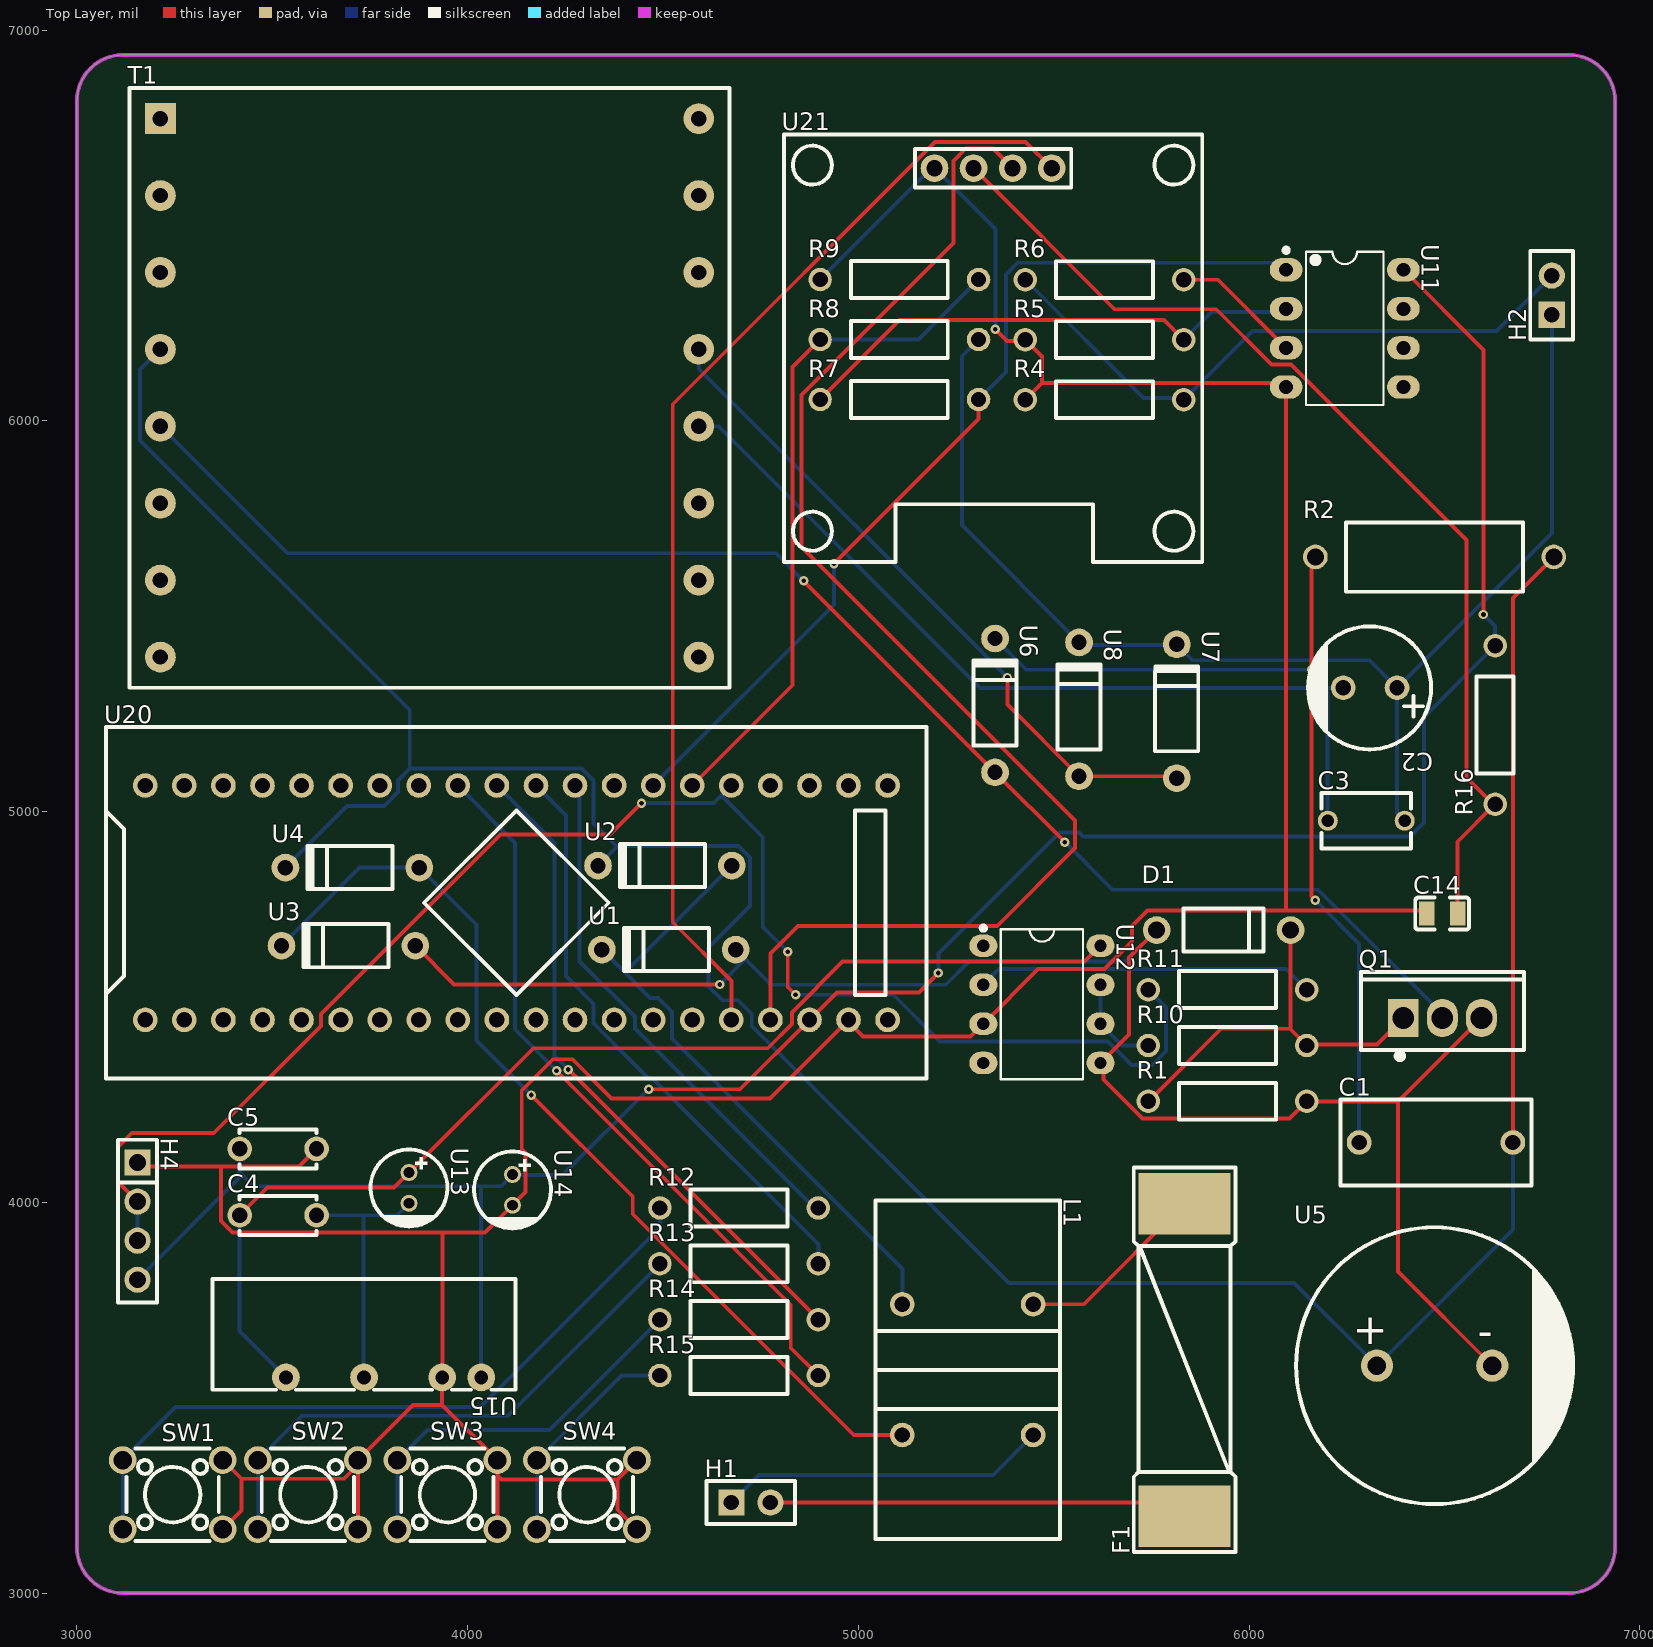
[diagram p0: Top Layer view]
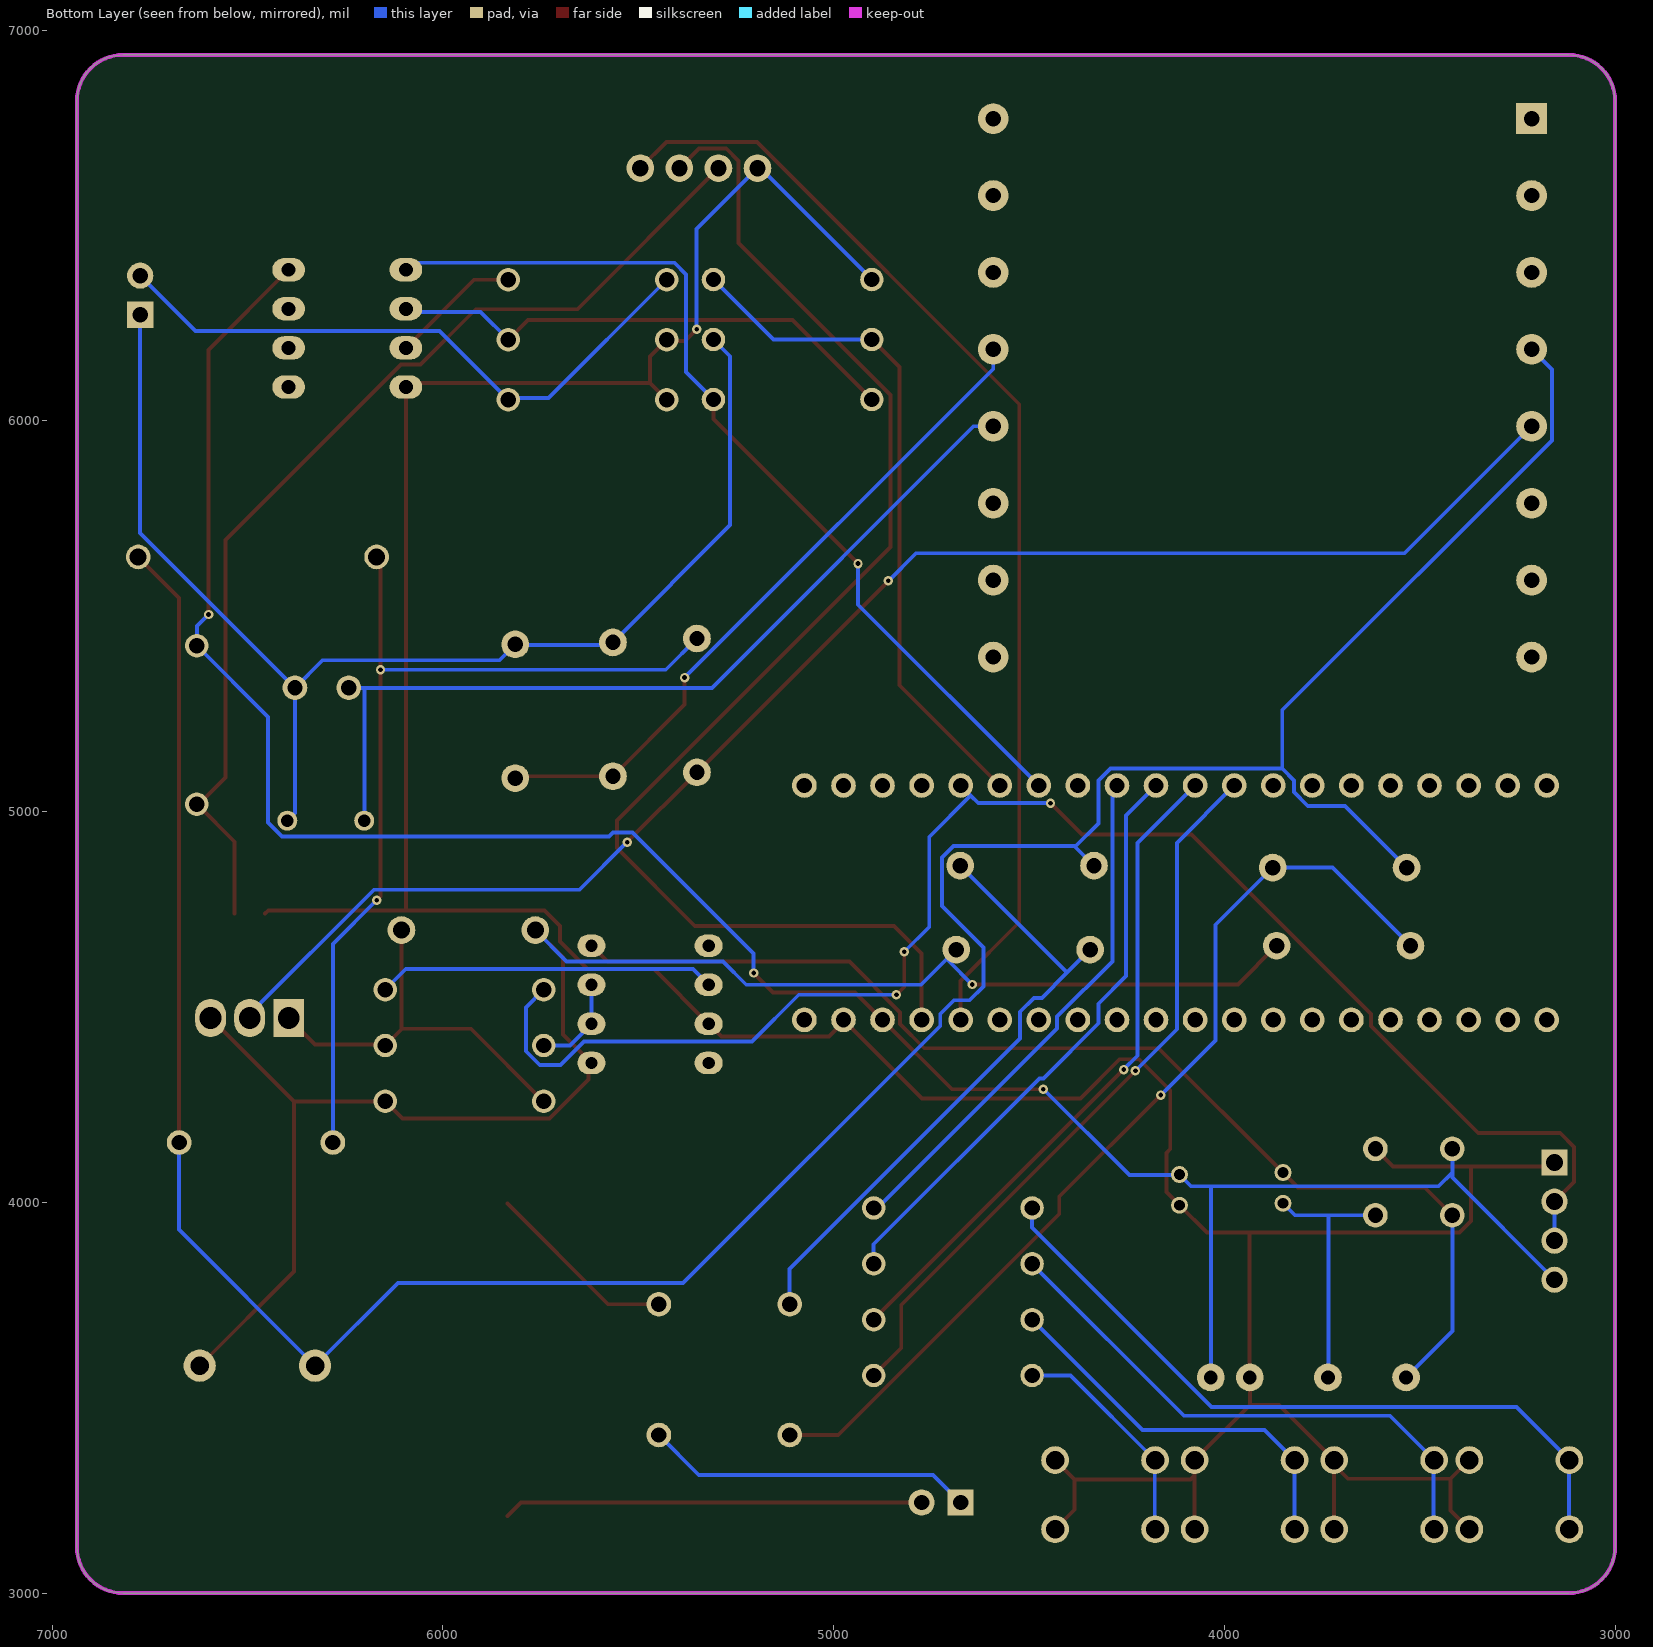
[diagram p1: Bottom Layer view, seen from below]
# Altium PCB MISC75075.pcbdoc
Units mil, origin at the board's own origin, x right, y up, seen from the top; angles counter-clockwise.
Board outline 3937.01 x 3937.01 mil, 2 copper layers (Top Layer, Bottom Layer), stack 62.206 mil thick; 48 components, 60 nets, 177 pads, 17 vias.

## Layer stack, top to bottom
Top Solder Mask Layer: solder mask 0.394, Dk 3.3
Top Layer: signal copper 1.379
Dielectric1: surface 59.449, FR4, Dk 4.5
Bottom Layer: signal copper 1.378
Bottom Solder Mask Layer: solder mask 0.394, Dk 3.3

## Board outline
3118.11,6937.01 ccw(c3118.11,6818.9) 3000,6818.9 3000,3118.11 ccw(c3118.11,3118.11) 3118.11,3000 6818.9,3000 ccw(c6818.9,3118.11) 6937.01,3118.11 6937.01,6818.9 ccw(c6818.9,6818.9) 6818.9,6937.01 3118.11,6937.01

## Design rules (kind name [scope] priority, off if disabled: settings)
BoardOutlineClearance copperThickness2oz_1 [All] p2 off: genericclearance=7.99 ignorepadtopadclearanceinfootprint=FALSE except(0: Arc-SplitContinuation Track-SplitContinuation SMDPad-SplitContinuation THPad-SplitContinuation Via-SplitContinuation Fill-SplitContinuation Region-SplitContinuation Poly-SplitContinuation Text-SplitContinuation Hole-SplitContinuation; 5.98: Arc-CutoutEdge Track-CutoutEdge SMDPad-CutoutEdge THPad-CutoutEdge Via-CutoutEdge Text-CutoutEdge; 6.9: Hole-OutlineEdge Hole-CutoutEdge; 10: Poly-OutlineEdge Poly-CutoutEdge; 11.81: Arc-OutlineEdge Track-OutlineEdge SMDPad-OutlineEdge THPad-OutlineEdge Via-OutlineEdge Fill-OutlineEdge Region-OutlineEdge Text-OutlineEdge Fill-CutoutEdge Region-CutoutEdge)
BoardOutlineClearance Plane_innerPlane_1 [All] p4 off: genericclearance=4.02 ignorepadtopadclearanceinfootprint=FALSE except(0: Arc-SplitContinuation Track-SplitContinuation SMDPad-SplitContinuation THPad-SplitContinuation Via-SplitContinuation Fill-SplitContinuation Region-SplitContinuation Poly-SplitContinuation Text-SplitContinuation Hole-SplitContinuation; 5.98: Arc-CutoutEdge Track-CutoutEdge SMDPad-CutoutEdge THPad-CutoutEdge Via-CutoutEdge Text-CutoutEdge; 6.9: Hole-OutlineEdge Hole-CutoutEdge; 10: Poly-OutlineEdge Poly-CutoutEdge; 11.81: Arc-OutlineEdge Track-OutlineEdge SMDPad-OutlineEdge THPad-OutlineEdge Via-OutlineEdge Fill-OutlineEdge Region-OutlineEdge Text-OutlineEdge Fill-CutoutEdge Region-CutoutEdge)
BoardOutlineClearance Copper_copperRegion_1 [All] p6 off: genericclearance=4.02 ignorepadtopadclearanceinfootprint=FALSE except(0: Arc-SplitContinuation Track-SplitContinuation SMDPad-SplitContinuation THPad-SplitContinuation Via-SplitContinuation Fill-SplitContinuation Region-SplitContinuation Poly-SplitContinuation Text-SplitContinuation Hole-SplitContinuation; 5.98: Arc-CutoutEdge Track-CutoutEdge SMDPad-CutoutEdge THPad-CutoutEdge Via-CutoutEdge Text-CutoutEdge; 6.9: Hole-OutlineEdge Hole-CutoutEdge; 10: Poly-OutlineEdge Poly-CutoutEdge; 11.81: Arc-OutlineEdge Track-OutlineEdge SMDPad-OutlineEdge THPad-OutlineEdge Via-OutlineEdge Fill-OutlineEdge Region-OutlineEdge Text-OutlineEdge Fill-CutoutEdge Region-CutoutEdge)
BoardOutlineClearance copperThickness1oz_1 [All] p8: genericclearance=4.02 ignorepadtopadclearanceinfootprint=FALSE except(0: Arc-SplitContinuation Track-SplitContinuation SMDPad-SplitContinuation THPad-SplitContinuation Via-SplitContinuation Fill-SplitContinuation Region-SplitContinuation Poly-SplitContinuation Text-SplitContinuation Hole-SplitContinuation; 5.98: Arc-CutoutEdge Track-CutoutEdge SMDPad-CutoutEdge THPad-CutoutEdge Via-CutoutEdge Text-CutoutEdge; 6.9: Hole-OutlineEdge Hole-CutoutEdge; 10: Poly-OutlineEdge Poly-CutoutEdge; 11.81: Arc-OutlineEdge Track-OutlineEdge SMDPad-OutlineEdge THPad-OutlineEdge Via-OutlineEdge Fill-OutlineEdge Region-OutlineEdge Text-OutlineEdge Fill-CutoutEdge Region-CutoutEdge)
Clearance copperThickness2oz [All] p1 off: gap=7.99 ignorepadtopadclearanceinfootprint=FALSE except(5.98: SMDPad-Track SMDPad-SMDPad THPad-Track SMDPad-THPad THPad-THPad Track-Via SMDPad-Via THPad-Via Via-Via Fill-SMDPad Region-SMDPad Fill-THPad Region-THPad Fill-Via Region-Via Fill-Fill Fill-Region Region-Region Arc-Track Arc-SMDPad Arc-THPad Arc-Via Fill-Arc Region-Arc Arc-Arc Text-Track SMDPad-Text Text-THPad Text-Via Fill-Text Region-Text Arc-Text Text-Text; 6.9: Hole-Track Hole-SMDPad Hole-THPad Hole-Via Fill-Hole Region-Hole Hole-Arc Hole-Text; 10: Poly-Track Poly-SMDPad Poly-THPad Poly-Via Poly-Fill Poly-Region Poly-Poly Poly-Arc Poly-Text Poly-Hole; 11.81: Fill-Track Region-Track)
Clearance Plane_innerPlane [All] p3 off: gap=4.02 ignorepadtopadclearanceinfootprint=FALSE except(5.98: SMDPad-Track SMDPad-SMDPad THPad-Track SMDPad-THPad THPad-THPad Track-Via SMDPad-Via THPad-Via Via-Via Fill-SMDPad Region-SMDPad Fill-THPad Region-THPad Fill-Via Region-Via Fill-Fill Fill-Region Region-Region Arc-Track Arc-SMDPad Arc-THPad Arc-Via Fill-Arc Region-Arc Arc-Arc Text-Track SMDPad-Text Text-THPad Text-Via Fill-Text Region-Text Arc-Text Text-Text; 6.9: Hole-Track Hole-SMDPad Hole-THPad Hole-Via Fill-Hole Region-Hole Hole-Arc Hole-Text; 10: Poly-Track Poly-SMDPad Poly-THPad Poly-Via Poly-Fill Poly-Region Poly-Poly Poly-Arc Poly-Text Poly-Hole; 11.81: Fill-Track Region-Track)
Clearance Copper_copperRegion [All] p5 off: gap=4.02 ignorepadtopadclearanceinfootprint=FALSE except(5.98: SMDPad-Track SMDPad-SMDPad THPad-Track SMDPad-THPad THPad-THPad Track-Via SMDPad-Via THPad-Via Via-Via Fill-SMDPad Region-SMDPad Fill-THPad Region-THPad Fill-Via Region-Via Fill-Fill Fill-Region Region-Region Arc-Track Arc-SMDPad Arc-THPad Arc-Via Fill-Arc Region-Arc Arc-Arc Text-Track SMDPad-Text Text-THPad Text-Via Fill-Text Region-Text Arc-Text Text-Text; 6.9: Hole-Track Hole-SMDPad Hole-THPad Hole-Via Fill-Hole Region-Hole Hole-Arc Hole-Text; 10: Poly-Track Poly-SMDPad Poly-THPad Poly-Via Poly-Fill Poly-Region Poly-Poly Poly-Arc Poly-Text Poly-Hole; 11.81: Fill-Track Region-Track)
Clearance copperThickness1oz [All] p7: gap=4.02 ignorepadtopadclearanceinfootprint=FALSE except(5.98: SMDPad-Track SMDPad-SMDPad THPad-Track SMDPad-THPad THPad-THPad Track-Via SMDPad-Via THPad-Via Via-Via Fill-SMDPad Region-SMDPad Fill-THPad Region-THPad Fill-Via Region-Via Fill-Fill Fill-Region Region-Region Arc-Track Arc-SMDPad Arc-THPad Arc-Via Fill-Arc Region-Arc Arc-Arc Text-Track SMDPad-Text Text-THPad Text-Via Fill-Text Region-Text Arc-Text Text-Text; 6.9: Hole-Track Hole-SMDPad Hole-THPad Hole-Via Fill-Hole Region-Hole Hole-Arc Hole-Text; 10: Poly-Track Poly-SMDPad Poly-THPad Poly-Via Poly-Fill Poly-Region Poly-Poly Poly-Arc Poly-Text Poly-Hole; 11.81: Fill-Track Region-Track)
DiffPairsRouting differentialPair [All] p1: maxlimit=6 minlimit=6 mostfreqgap=6 toplayer_minwidth=5 toplayer_prefwidth=10 toplayer_maxwidth=100 toplayer_mingap=6 toplayer_prefgap=6 toplayer_maxgap=6 bottomlayer_minwidth=5 bottomlayer_prefwidth=10 bottomlayer_maxwidth=100 bottomlayer_mingap=6 bottomlayer_prefgap=6 bottomlayer_maxgap=6 maxuncoupledlength=10
HoleToHoleClearance otherClearance [All] p1: gap=11.81 allowstackedmicrovias=TRUE
Length netLength [All] p1: minlimit=0 maxlimit=0
PasteMaskExpansion pasteMaskExpansion [All] p1: expansion=0
PlaneConnect innerPlane [All] p1: planeconnectstyle=Relief reliefexpansion=20 reliefentries=4 reliefconductorwidth=10 reliefairgap=10
PolygonConnect copperRegion [All] p1: connectstyle=Relief reliefconductorwidth=10 reliefentries=4 polygonreliefangle="90 Angle" airgapwidth=10 via.connectstyle=Relief via.reliefconductorwidth=10 via.reliefentries=4 via.polygonreliefangle="90 Angle" via.airgapwidth=10
RoutingVias viaSize [All] p1: holewidth=12.01 width=24.02 viastyle="Through Hole" minholewidth=11.81 minwidth=19.68 maxholewidth=248.03 maxwidth=393.7
SolderMaskExpansion solderMaskExpansion [IsVia] p1: expansion=-1000 istentingtop=TRUE
SolderMaskExpansion solderMaskExpansion [All] p2: expansion=2 istentingtop=FALSE
Width copperThickness2oz_2 [All] p1 off: maxlimit=100 minlimit=8 preferedwidth=10
Width copperThickness1oz_2 [All] p2: maxlimit=100 minlimit=5 preferedwidth=10

## Components (designator, comment, footprint, x,y, rotation, side; value= is the part's Value field where it differs from the comment)
C1 "100uF" CAP-TH_L12.0-W5.5-P10.00-D1.0 6478.63,4153.38 r0 top
C2 "220uF" CAP-TH_BD8.0-P3.50-D0.6-FD 6310,5317.01 r180 top
C3 "1uF" CAP-TH_L5.8-W3.6-P5.0-D0.6 6300,4977.01 r0 top
C4 "100nF" CAP-TH_L5.0-W2.5-P5.00-D1.0 3515,3967.01 r0 top
C5 "100nF" CAP-TH_L5.0-W2.5-P5.00-D1.0 3515,4137.01 r0 top
C14 "100nF" C0805 6494.43,4739.12 r0 top
D1 "1N4742" DO-41_BD2.4-L4.7-P8.70-D0.8-FD 5935,4697.01 r0 top
F1 "5F.2000210000R1" FUSE-SMD_5-20MM 5835,3597.01 r90 top
H1 "" HDR-TH_2P-P2.54-V-F 4725,3232.01 r0 top
H2 "" HDR-TH_2P-P2.54-V-F 6775,6322.01 r90 top
H4 "" HDR-TH_4P-P2.54-V-F 3155,3952.01 r270 top
L1 "PDMCAT18107-103ML" IND-TH_4P-L22.0-W12.0-TR 5280,3572.01 r270 top
Q1 "FQPF8N60C" TO-220F-3_L10.2-W4.9-P2.54-L 6495,4472.01 r0 top
R1 "10kΩ" Res_1/4W 5945,4258.67 r0 top
R2 "10kΩ" Res_1W 6475,5652.01 r0 top
R4 "10mΩ" Res_1/4W 5630,6054.51 r0 top
R5 "2kΩ" Res_1/4W 5630,6208.01 r0 top
R6 "2kΩ" Res_1/4W 5630,6361.51 r0 top
R7 "200kΩ" Res_1/4W 5105,6055.01 r0 top
R8 "10kΩ" Res_1/4W 5105,6208.51 r0 top
R9 "2kΩ" Res_1/4W 5105,6362.01 r0 top
R10 "10Ω" Res_1/4W 5945,4401.59 r0 top
R11 "1kΩ" Res_1/4W 5945,4544.51 r0 top
R12 "2kΩ" Res_1/4W 4695,3985.76 r0 top
R13 "2kΩ" Res_1/4W 4695,3842.84 r0 top
R14 "2kΩ" Res_1/4W 4695,3699.92 r0 top
R15 "2kΩ" Res_1/4W 4695,3557.01 r0 top
R16 "1kΩ" Res_1/4W 6630,5222.01 r90 top
SW1 "TS-1002-07026" SW-TH_4P-L6.0-W6.0-P4.50-LS6.5 3245,3252.01 r0 top
SW2 "TS-1002-07026" SW-TH_4P-L6.0-W6.0-P4.50-LS6.5 3591.17,3252.01 r0 top
SW3 "TS-1002-07026" SW-TH_4P-L6.0-W6.0-P4.50-LS6.5 3948.33,3252.01 r0 top
SW4 "TS-1002-07026" SW-TH_4P-L6.0-W6.0-P4.50-LS6.5 4305.5,3252.01 r0 top
T1 "" dip2_8_5mm_35MM 3135,6577.01 r0 top
U1 "1N4007" DO-41_BD2.4-L4.7-P8.70-D0.6-RD 4515,4647.01 r0 top
U2 "1N4007" DO-41_BD2.4-L4.7-P8.70-D0.6-RD 4505,4862.01 r0 top
U3 "1N4007" DO-41_BD2.4-L4.7-P8.70-D0.6-RD 3695,4657.01 r0 top
U4 "1N4007" DO-41_BD2.4-L4.7-P8.70-D0.6-RD 3705,4857.01 r0 top
U5 "150uF" CAP-TH_BD18.0-P7.50-D0.8-FD 6475,3582.01 r0 top
U6 "1N4007" DO-41_BD2.4-L4.7-P8.70-D0.6-RD 5350,5272.01 r270 top
U7 "1N4007" DO-41_BD2.4-L4.7-P8.70-D0.6-RD 5815,5257.01 r270 top
U8 "1N4007" DO-41_BD2.4-L4.7-P8.70-D0.6-RD 5565,5262.01 r270 top
U11 "LM358" DIP-8_L9.8-W6.4-P2.54-LS7.6-BL 6245,6237.01 r270 top
U12 "TLP250(F)" DIP-8_L9.4-W6.4-P2.54-LS9.1-BL 5470,4507.01 r270 top
U13 "47uF" CAP-TH_BD5.0-P2.00-D0.5-FD 3850,4037.01 r270 top
U14 "100uF" CAP-TH_BD5.0-P2.00-D0.5-FD 4115,4032.01 r270 top
U15 "B0515S-2WR3" SIP-4_L19.5-W7.0-P2.54-L 3785,3552.01 r180 top
U20 "LCKFB-DKX-STM32F103C8T6" CONN-TH_L53.3-W22.9_STM32F103C8T6-CARD 4125,4767.01 r0 top
U21 "HS96L03W2C03" OLED-TH_L27.8-W27.2-P2.54_C9900033791 5345,6647.01 r0 top

## Footprints (in the part's own frame and the unit in brackets; to place one, negate y for a bottom-side part, rotate by r counter-clockwise, add the part's x,y. Pads: shape width x height; smd on the part's side, far side on the other; paste and mask are expansions set on the pad)
C0805 [mm]
  rect 1x1.55 smd paste+0 mask+0.102: 1(-1,0) 2(1,0)
  silkscreen extent -1.75,-1.04 1.75,1.04
CAP-TH_BD5.0-P2.00-D0.5-FD [mm]
  round 1.1 hole 0.7 paste+0 mask+0.05: 1(-1,0) 2(1,0)
  silkscreen extent -2.5,-2.5 2.5,2.5
CAP-TH_BD8.0-P3.50-D0.6-FD [mm]
  round 1.6 hole 1: 1(-1.75,0) 2(1.75,0)
  silkscreen extent -3.96,-4 4.04,4
CAP-TH_BD18.0-P7.50-D0.8-FD [mm]
  round 2.1 hole 1.2 paste+0 mask+0.05: 1(-3.75,0) 2(3.75,0)
  silkscreen extent -9,-9 9,9
CAP-TH_L5.0-W2.5-P5.00-D1.0 [mm]
  round 1.6 hole 1: 1(-2.5,0) 2(2.5,0)
  silkscreen extent -2.5,-1.27 2.5,1.25
CAP-TH_L5.8-W3.6-P5.0-D0.6 [mm]
  round 1.3 hole 0.8 paste+0 mask+0.05: 1(-2.5,0)
  round 1.3 hole 0.8 copper offset 0,0 paste+0 mask+0.05: 2(2.5,0)
  silkscreen extent -2.9,-1.8 2.9,1.8
CAP-TH_L12.0-W5.5-P10.00-D1.0 [mm]
  round 1.6 hole 1: 1(-5,0) 2(5,0)
  silkscreen extent -6.2,-2.8 6.2,2.8
CONN-TH_L53.3-W22.9_STM32F103C8T6-CARD [mm]
  round 1.6 hole 1: 1(-24.13,-7.62) 2(-21.59,-7.62) 3(-19.05,-7.62) 4(-16.51,-7.62) 5(-13.97,-7.62) 6(-11.43,-7.62) 7(-8.89,-7.62) 8(-6.35,-7.62) 9(-3.81,-7.62) 10(-1.27,-7.62) 11(1.27,-7.62) 12(3.81,-7.62) 13(6.35,-7.62) 14(8.89,-7.62) 15(11.43,-7.62) 16(13.97,-7.62) 17(16.51,-7.62) 18(19.05,-7.62) 19(21.59,-7.62) 20(24.13,-7.62) 21(24.13,7.62) 22(21.59,7.62) 23(19.05,7.62) 24(16.51,7.62) 25(13.97,7.62) 26(11.43,7.62) 27(8.89,7.62) 28(6.35,7.62) 29(3.81,7.62) 30(1.27,7.62) 31(-1.27,7.62) 32(-3.81,7.62) 33(-6.35,7.62) 34(-8.89,7.62) 35(-11.43,7.62) 36(-13.97,7.62) 37(-16.51,7.62) 38(-19.05,7.62) 39(-21.59,7.62) 40(-24.13,7.62)
  silkscreen extent -26.67,-11.43 26.67,11.43
dip2_8_5mm_35MM [mm]
  rect 2x2 hole 1: 1(2,5)
  round 2 hole 1: 2(2,0) 3(2,-5) 4(2,-10) 5(2,-15) 6(2,-20) 7(2,-25) 8(2,-30) 9(37,5) 10(37,0) 11(37,-5) 12(37,-10) 13(37,-15) 14(37,-20) 15(37,-25) 16(37,-30)
  silkscreen extent 0,-32 39,7
DIP-8_L9.4-W6.4-P2.54-LS9.1-BL [mm]
  oval 1.46x1.825 hole 0.8: 1(-3.81,-3.81) 2(-1.27,-3.81) 3(1.27,-3.81) 4(3.81,-3.81) 5(3.81,3.81) 6(1.27,3.81) 7(-1.27,3.81) 8(-3.81,3.81)
  silkscreen extent -5.1,-3.96 4.87,2.67
DIP-8_L9.8-W6.4-P2.54-LS7.6-BL [mil]
  oval 60x83.66 hole 35.43: 1(-150,-150) 2(-50,-150) 3(50,-150) 4(150,-150) 5(150,150) 6(50,150) 7(-50,150) 8(-150,150)
  silkscreen extent -206,-156 196,99
DO-41_BD2.4-L4.7-P8.70-D0.6-RD [mm]
  round 1.8 hole 1: 1(-4.35,0) 2(4.35,0)
  silkscreen extent -2.92,-1.4 2.6,1.4
DO-41_BD2.4-L4.7-P8.70-D0.8-FD [mm]
  round 1.8 hole 1.1: 1(-4.35,0) 2(4.35,0)
  silkscreen extent -2.6,-1.4 2.6,1.4
FUSE-SMD_5-20MM [mm]
  rect 4x6 smd: 1(-10.16,0) 2(10.16,0)
  silkscreen extent -12.5,-3.3 12.5,3.3
HDR-TH_2P-P2.54-V-F [mm]
  rect 1.7x1.7 hole 1: 1(-1.27,0)
  round 1.7 hole 1: 2(1.27,0)
  silkscreen extent -2.88,-1.39 2.88,1.4
HDR-TH_4P-P2.54-V-F [mm]
  rect 1.7x1.7 hole 1.1: 1(-3.81,0)
  round 1.7 hole 1.1: 2(-1.27,0) 3(1.27,0) 4(3.81,0)
  silkscreen extent -5.29,-1.27 5.29,1.27
IND-TH_4P-L22.0-W12.0-TR [mm]
  round 1.6 hole 1 paste+0 mask+0.05: 1(4.25,4.25) 2(4.25,-4.25) 3(-4.25,-4.25) 4(-4.25,4.25)
  silkscreen extent -11,-6.01 11,6
OLED-TH_L27.8-W27.2-P2.54_C9900033791 [mm]
  round 1.8 hole 1.05 paste+0 mask+0.05: 1(-3.81,0) 2(-1.27,0) 3(1.27,0) 4(3.81,0)
  silkscreen extent -13.6,-25.6 13.6,2.2
Res_1/4W [mil]
  round 60 hole 39.37 paste+0 mask+2: 1(-202.76,0) 2(202.76,0)
  silkscreen extent -124,-47 124,47
Res_1W [mm]
  round 1.6 hole 1.1 paste+0 mask+0.051: 1(-7.75,0) 2(7.75,0)
  silkscreen extent -5.75,-2.26 5.75,2.25
SIP-4_L19.5-W7.0-P2.54-L [mm]
  round 1.8 hole 0.9 paste+0 mask+0.05: 1(-6.35,0) 2(-3.81,0) 4(1.27,0) 6(6.35,0)
  silkscreen extent -8.58,-6.4 11.12,0.8
SW-TH_4P-L6.0-W6.0-P4.50-LS6.5 [mm]
  round 1.8 hole 1.2: 1(-3.25,2.25) 2(3.25,2.25) 3(-3.25,-2.25) 4(3.25,-2.25)
  silkscreen extent -3,-3 3,3
TO-220F-3_L10.2-W4.9-P2.54-L [mm]
  rect 2x2.5 hole 1.4: 1(-2.54,0)
  oval 2x2.5 hole 1.4: 2(0,0) 3(2.54,0)
  silkscreen extent -5.3,-2.66 5.3,3

## Via types
v1: diameter 24.02, hole 12, Top Layer to Bottom Layer, 17 vias

## Nets (pads, with @x,y where several pads share a name; then routed paths per layer and width w, separated by ;. In a path a pad name is that pad's centre, name@x,y a point inside that pad or via, vN(x,y) a via of type N, cw(c..) or ccw(c..) an arc to the next point about the centre after c; other vN are vias at no path point)
3.3V: U20.20
310VDC: C1.2 R2.2 T1.4 U2.1 U4.1 U5.1 | length 7682.1
  Top Layer w10: C1.2 6675.48,5547.37 R2.2
  Bottom Layer w10: T1.4 3161.97,6131.54 3161.97,5950.24 3851.97,5260.24 3851.97,5110.24 ; U4.1 3691.62,5014.88 3786.62,5014.88 3821.97,5050.24 3821.97,5080.24 3851.97,5110.24 ; U2.1 4381.97,4910.24 ; C1.2 6675.48,3930.13 U5.1 6115.23,3794.14 5385.23,3794.14 4727.36,4452.01 4727.36,4482.01 4692,4517.36 4652,4517.36 4616.65,4552.72 4616.65,4652.72 4722.72,4758.78 4722.72,4883.03 4693.74,4912.01 4383.74,4912.01 4381.97,4910.24 ; 3851.97,5110.24 4291.97,5110.24 4321.97,5080.24 4321.97,4970.24 4381.97,4910.24
$1N2604: L1.3 U1.1 U2.2 | length 1625.8
  Bottom Layer w10: U1.1 4403.69,4587.06 ; U2.2 4403.69,4589.43 4403.69,4587.06 ; L1.3 5112.68,3829.33 4522.68,4419.33 4522.68,4488.07 4487.32,4523.42 4467.32,4523.42 4403.69,4587.06
$1N2605: L1.2 U3.1 U4.2 | length 2472.6
  Top Layer w10: v1(4162.68,4274.69) 4422.76,4014.61 4422.76,3970.37 4988.44,3404.69 L1.2
  Bottom Layer w10: U3.1 3723.74,4857.01 U4.2 4022.68,4710.59 4022.68,4414.69 v1(4162.68,4274.69)
$1N2608: H1.1 L1.1 | length 843.8
  Bottom Layer w10: H1.1 4745.71,3302.72 5345.35,3302.72 L1.1
$1N2611: Q1.2 T1.5 U6.2 | length 3914.4
  Top Layer w10: v1(4860,5590.75) U6.2 v1(5528.74,4922.01)
  Bottom Layer w10: T1.5 3538.74,5661.46 4789.29,5661.46 v1(4860,5590.75) ; v1(5528.74,4922.01) 5650.54,4800.21 6176.8,4800.21 6495,4482.01 Q1.2
$1N2613: C1.1 R2.1 U6.1 | length 2396.2
  Top Layer w10: v1(6169.88,4773.38) 6159.88,4783.38 v1(6159.88,5363.38) 6159.88,5642.01 R2.1
  Bottom Layer w10: U6.1 5429.89,5363.38 v1(6159.88,5363.38) ; v1(6169.88,4773.38) 6281.78,4661.47 C1.1
$1N2616: T1.12 U7.2 U8.2 | length 1747.8
  Top Layer w10: v1(5381.69,5343.31) 5381.69,5274.06 U8.2 5810,5090.75 U7.2
  Bottom Layer w10: T1.12 4591.69,6133.31 v1(5381.69,5343.31)
$1N2617: C2.2 C3.1 T1.13 | length 2266.9
  Bottom Layer w10: T1.13 4641.69,5986.46 5311.14,5317.01 6201.14,5317.01 ; C3.1 6201.14,4977.44 6201.14,5317.01 ; C2.2 6201.14,5317.01
$1N2621: H2.2 R4.2 R6.1 | length 1609.1
  Bottom Layer w10: R6.1 5729.63,6059.11 R4.2@5837.37,6059.11 ; R4.2 R4.2@5837.37,6059.11 ; H2.2 6633.58,6230.59 6008.84,6230.59 R4.2@5837.37,6059.11
$1N2626: R5.2 R7.1 U11.2 | length 1330.3
  Top Layer w10: R7.1 5105.24,6258.01 5782.76,6258.01 R5.2
  Bottom Layer w10: R5.2 5903.47,6278.72 6086.71,6278.72 U11.2
$1N2629: R6.2 U11.3 | length 334.5
  Top Layer w10: R6.2 5920.5,6361.51 U11.3
$1N2637: R10.1 U12.6 U12.7 | length 245.2
  Bottom Layer w10: U12.7 U12.6 5675.42,4401.59 R10.1
$1N2638: R11.2 U12.2 | length 866.1
  Bottom Layer w10: U12.2 5360,4597.01 6095.26,4597.01 R11.2
$1N2639: C4.2 U13.2 U15.4 | length 664.9
  Bottom Layer w10: C4.2 3733.43,3967.01 ; U15.4 3733.43,3553.58 3733.43,3967.01 ; U13.2 3819.37,3967.01 3733.43,3967.01
$1N5745: R12.1 SW1.1 SW1.3 | length 1850.6
  Bottom Layer w10: SW1.3 3118.25,3164.63 SW1.1@3118.25,3341.79 ; SW1.1 SW1.1@3118.25,3341.79 ; R12.1 4492.24,3935.76 4032.62,3476.14 3252.6,3476.14 SW1.1@3118.25,3341.79
$1N5869: R13.1 SW2.1 SW2.3 | length 1417
  Bottom Layer w10: SW2.3 3465.19,3165.4 SW2.1@3465.19,3342.56 ; SW2.1 SW2.1@3465.19,3342.56 ; R13.1 4103.33,3453.93 3576.56,3453.93 SW2.1@3465.19,3342.56
$1N5889: R15.1 SW4.1 SW4.3 | length 582.6
  Bottom Layer w10: SW4.3 4178.3,3164.18 SW4.1@4178.3,3341.34 ; SW4.1 SW4.1@4178.3,3341.34 ; R15.1 4393.97,3557.01 SW4.1@4178.3,3341.34
$1N5921: R14.1 SW3.1 SW3.3 | length 998.5
  Bottom Layer w10: SW3.3 3820.86,3163.91 SW3.1@3820.86,3341.07 ; SW3.1 SW3.1@3820.86,3341.07 ; R14.1 4209.4,3417.08 3896.88,3417.08 SW3.1@3820.86,3341.07
$1N8200: C14.2 R16.1 U21.2 | length 2683.8
  Top Layer w10: U21.2 5656.07,6285.94 5916.07,6285.94 6057.49,6144.52 6107.49,6144.52 6556.78,5695.23 6556.78,5087.45 R16.1@6627.49,5016.73 ; C14.2 6533.8,4923.04 R16.1@6627.49,5016.73 ; R16.1@6630,5019.25 R16.1@6627.49,5016.73
$1N8407: F1.2 L1.4 | length 494.4
  Top Layer w10: L1.4 5577.32,3739.33 F1.2
$1N8411: F1.1 H1.2 | length 1074.5
  Top Layer w10: H1.2 5800,3232.01 F1.1
+5V: C5.1 H4.4 R16.2 U11.8 U14.1 U15.1 U20.18 | length 5991.8
  Top Layer w10: v1(4463.28,4289.66) 4697.66,4289.66 U20.18 4945.71,4537.72 5155.71,4537.72 v1(5205,4587.01) ; U11.8 6600,6182.01 v1(6600,5504.77)
  Bottom Layer w10: H4.4 3416.57,4063.58 3416.57,4077.01 ; C5.1 3416.57,4077.01 ; U15.1 4034.7,3552.3 4034.7,4041.38 ; U14.1 U14.1@4113.28,4069.66 ; v1(4463.28,4289.66) 4243.28,4069.66 U14.1@4113.28,4069.66 ; v1(5205,4587.01) 5205,4637.01 5515,4947.01 5565,4947.01 5575,4937.01 6412.24,4937.01 6447.6,4972.36 6447.6,5242.36 R16.2 6630,5474.77 v1(6600,5504.77) ; 3416.57,4077.01 3452.2,4041.38 4034.7,4041.38 ; 4034.7,4041.38 4085,4041.38 U14.1@4113.28,4069.66
AGND: D1.1 Q1.3 R1.2 U1.2 U3.2 U5.2 U12.5 | length 4429.4
  Top Layer w10: U3.2 3965.55,4557.72 v1(4645.55,4557.72) ; U12.5 U12.5@5627.62,4364.63 ; D1.1 5693.03,4626.3 5693.03,4430.04 U12.5@5627.62,4364.63 ; Q1.3 6381.67,4258.67 ; U5.2 6381.67,3822.98 6381.67,4258.67 ; U12.5@5627.62,4364.63 5627.62,4314.63 5727.62,4214.63 6103.72,4214.63 R1.2 6381.67,4258.67
  Bottom Layer w10: v1(4645.55,4557.72) 4705.55,4617.72 U1.2@4705.55,4627.72 ; U1.2 U1.2@4705.55,4627.72 ; D1.1 5683.74,4617.01 5283.74,4617.01 5223.74,4557.01 4776.26,4557.01 U1.2@4705.55,4627.72
G: D1.2 Q1.1 R1.1 R10.2 | length 1031.5
  Top Layer w10: R1.1 5928.07,4444.51 6106.26,4444.51 ; D1.2 6106.26,4444.51 ; R10.2 R10.2@6145.15,4404.2 ; Q1.1 6327.19,4404.2 R10.2@6145.15,4404.2 ; 6106.26,4444.51 6106.26,4443.09 R10.2@6145.15,4404.2
GND: C5.2 C14.1 H4.1 R4.1 R5.1 R9.1 SW1.2 SW1.4 SW2.2 SW2.4 SW3.2 SW3.4 SW4.2 SW4.4 U11.4 U12.3 U14.2 U15.2 U20.19 U21.1 | length 9855.6
  Top Layer w10: H4.1 3165,4092.01 3368.43,4092.01 ; SW1.4 3420.81,3211.28 3420.81,3292.73 ; SW1.2 3420.81,3292.73 ; C5.2 3568.43,4092.01 3368.43,4092.01 ; SW2.4 SW2.2@3719.12,3328.09 ; SW3.4 4076.28,3300.59 ; SW4.4@4433.45,3163.43 4383.45,3213.43 4383.45,3290.59 ; SW4.2@4433.45,3340.59 4383.45,3290.59 ; U20.19 U20.19@4972.26,4464.27 ; v1(5350.85,6234.4) 5380.85,6204.4 R5.1@5430.85,6204.4 ; R4.1 5469.74,6097.01 ; R5.1 R5.1@5430.85,6204.4 ; U11.4 U11.4@6095,6057.01 ; C14.1 6447.16,4747.01 6095,4747.01 ; 3368.43,4092.01 3368.43,3952.64 3398.43,3922.64 3935.93,3922.64 ; 3420.81,3292.73 3683.76,3292.73 SW2.2@3719.12,3328.09 ; SW2.2@3719.12,3328.09 SW2.2 3860.4,3481.87 3935,3481.87 ; 3935,3481.87 U15.2 3935.93,3552.93 3935.93,3922.64 ; 3935,3481.87 SW3.2 4076.28,3300.59 ; 3935.93,3922.64 4045,3922.64 U14.2 4148.64,4026.28 4148.64,4126.28 4138.64,4136.28 4138.64,4286.28 4218.64,4366.28 4268.64,4366.28 4368.64,4266.28 4774.27,4266.28 U20.19@4972.26,4464.27 ; 4076.28,3300.59 4086.28,3290.59 4383.45,3290.59 ; U20.19@4972.26,4464.27 5012.26,4424.27 5287.26,4424.27 U12.3 5460,4597.01 5630,4597.01 5700.71,4667.72 5700.71,4707.72 5740,4747.01 6095,4747.01 ; R5.1@5430.85,6204.4 5469.74,6165.51 5469.74,6097.01 ; 5469.74,6097.01 6055,6097.01 U11.4@6095,6057.01 ; 6095,4747.01 U11.4@6095,6057.01
  Bottom Layer w10: R9.1 5185.19,6644.95 U21.1@5197.05,6644.95 ; U21.1 U21.1@5197.05,6644.95 ; v1(5350.85,6234.4) 5350.85,6491.16 U21.1@5197.05,6644.95
KEY1: R12.2 U20.29 | length 1345.1
  Bottom Layer w10: U20.29 4286.72,5055.29 4286.72,4616.8 4428.14,4475.38 4428.14,4445.38 4887.76,3985.76 R12.2
KEY2: R13.2 U20.30 | length 1529.4
  Bottom Layer w10: U20.30 4251.36,4990.65 4251.36,4579.24 4322.07,4508.53 4322.07,4458.53 4463.5,4317.11 4473.5,4317.11 4897.76,3892.84 R13.2
KEY3: R14.2 U20.31 | length 1707.9
  Top Layer w10: v1(4257.76,4339.92) R14.2
  Bottom Layer w10: U20.31 4222.4,4919.61 4222.4,4375.28 v1(4257.76,4339.92)
KEY4: R15.2 U20.32 | length 1892.2
  Top Layer w10: v1(4227.76,4337.01) 4827.05,3737.72 4827.05,3627.72 R15.2
  Bottom Layer w10: U20.32 4121.69,4920.32 4121.69,4443.07 v1(4227.76,4337.01)
PA4: U20.28
PA8: U20.5
PA9: U20.6
PA10: U20.7
PA11: U20.8
PA12: U20.9
PA15: U20.10
PB0: U20.33
PB1: U20.34
PB3: U20.11
PB4: U20.12
PB5: U20.13
PB6: U20.14
PB7: U20.15
PB10: U20.35
PB11: U20.36
PB12: U20.1
PB13: U20.2
PB14: U20.3
PB15: U20.4
PC13: U20.22
PC14: U20.23
PC15: U20.24
PWM: H4.2 H4.3 R11.1 U20.25 | length 4034
  Top Layer w10: H4.2 3105,4052.01 3105,4142.01 3140.36,4177.36 3350.36,4177.36 3625,4452.01 3625,4482.01 4084.62,4941.63 4364.62,4941.63 v1(4445,5022.01) ; v1(4819.45,4641.45) 4819.45,4551.45 v1(4839.45,4531.45)
  Bottom Layer w10: H4.3 H4.2 ; v1(4445,5022.01) 4630,5022.01 4649.45,5041.45 ; U20.25 4649.45,5041.45 ; v1(4819.45,4641.45) 4755.51,4705.39 4755.51,4935.39 4649.45,5041.45 ; v1(4839.45,4531.45) 5089.45,4531.45 5209.45,4411.45 5639.19,4411.45 5699.19,4351.45 5752.24,4351.45 5787.6,4386.81 5787.6,4499.15 R11.1
SCL: U20.17 U21.3 | length 3456.5
  Top Layer w10: U20.17 4775,4637.01 4845.71,4707.72 5355.71,4707.72 5555,4907.01 5555,4977.01 4855,5677.01 4855,6067.01 5243.91,6455.92 5243.91,6665.92 5275,6697.01 5345,6697.01 U21.3
SDA: U20.16 U21.4 | length 2914.1
  Top Layer w10: U20.16 4675,4567.01 4525,4717.01 4525,6042.77 5196.75,6714.52 5427.48,6714.52 U21.4
UO_I_AD: R7.2 U11.1 U20.27 | length 2419.1
  Top Layer w10: v1(4937.76,5635.01) 5307.76,6005.01 R7.2
  Bottom Layer w10: U20.27 4937.76,5529.77 v1(4937.76,5635.01) ; R7.2 5377.76,6125.01 5377.76,6375.01 5407.76,6405.01 6077,6405.01 U11.1
UO_V_AD: R8.1 R9.2 U20.26 | length 1746.1
  Top Layer w10: U20.26 4831.53,5323.54 4831.53,6137.8 R8.1
  Bottom Layer w10: R8.1 5154.26,6208.51 R9.2
UOUT: C2.1 C3.2 H2.1 R8.2 U7.1 U8.1 | length 3248.8
  Bottom Layer w10: R8.2 5265,6165.75 5265,5733.27 U8.1 5571.66,5426.61 U7.1@5816.66,5426.61 ; U7.1 U7.1@5816.66,5426.61 ; C3.2 6378.9,4996.53 C2.1 ; H2.1 6775,5713.11 C2.1 ; U7.1@5816.66,5426.61 5855.55,5387.72 6308.19,5387.72 C2.1
VCC15V: C4.1 U12.8 U13.1 U15.6 | length 2970.9
  Top Layer w10: C4.1 3487.29,4037.72 3811.34,4037.72 U13.1 4168.2,4394.58 4768.2,4394.58 4830,4456.38 4830,4486.38 4960,4616.38 5579.37,4616.38 U12.8
  Bottom Layer w10: C4.1 3416.57,3670.43 U15.6
pads on no net: T1.1 T1.2 T1.3 T1.6 T1.7 T1.8 T1.9 T1.10 T1.11 T1.14 T1.15 T1.16 U11.5 U11.6 U11.7 U12.1 U12.4 U20.21 U20.37 U20.38 U20.39 U20.40

## Keep-outs
Board Outline Layer:
  the board outline again, w10